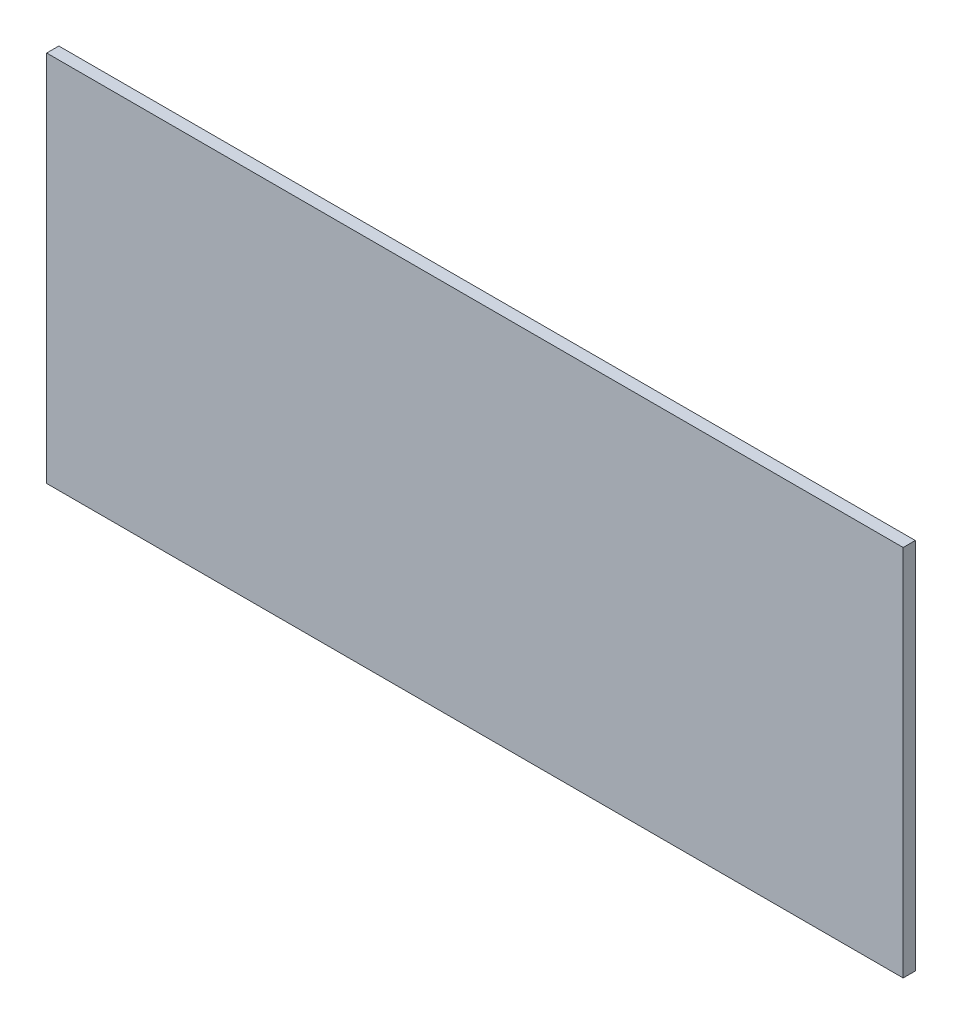
SolidWorks part; units mm, degrees
material "Q235"
ref_plane "Front Plane" through (0, 0, 0) normal (0, 0, 1) x (1, 0, 0)
ref_plane "Top Plane" through (0, 0, 0) normal (0, 1, 0) x (1, 0, 0)
ref_plane "Right Plane" through (0, 0, 0) normal (1, 0, 0) x (0, 0, -1)
sketch "Sketch1" plane through (0, 0, 0) normal (0, 0, 1) x (1, 0, 0)
  line L1 (0, 0) -> (2118, 0)
  line L2 (0, 0) -> (0, 922)
  line L3 (0, 922) -> (2118, 922)
  line L4 (2118, 0) -> (2118, 922)
  dimension "D1" = 2118
  dimension "D2" = 922
extrude "Boss-Extrude1" add sketch "Sketch1" along normal blind 30
